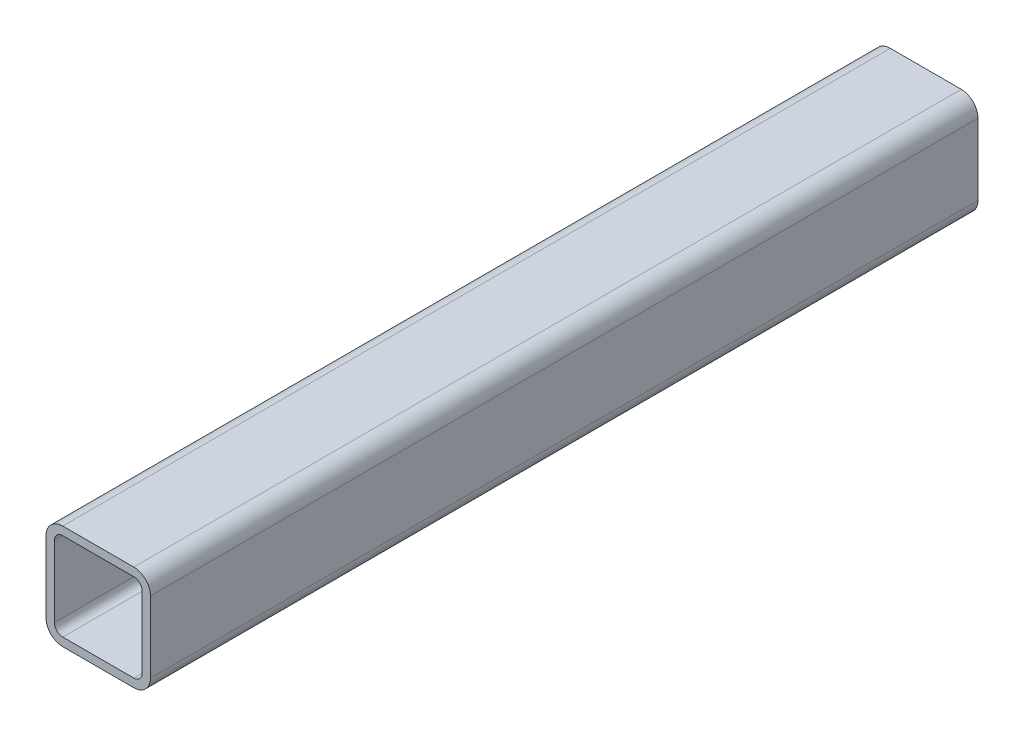
SolidWorks part; units mm, degrees
material "Q235"
ref_plane "Plane1" through (0, 0, 0) normal (0, 0, 1) x (1, 0, 0)
ref_plane "Plane2" through (0, 0, 0) normal (0, 1, 0) x (1, 0, 0)
ref_plane "Plane3" through (0, 0, 0) normal (1, 0, 0) x (0, 0, -1)
sketch "Sketch1" plane through (0, 0, 0) normal (0, 0, 1) x (1, 0, 0)
  line L0 (-8.5, -10.5) -> (8.5, -10.5)
  line L1 (-10.5, -8.5) -> (-10.5, 8.5)
  line L2 (8.5, 10.5) -> (-8.5, 10.5)
  line L3 (10.5, 8.5) -> (10.5, -8.5)
  line L4 (-8.5, -12.5) -> (8.5, -12.5)
  line L5 (-12.5, -8.5) -> (-12.5, 8.5)
  line L6 (8.5, 12.5) -> (-8.5, 12.5)
  line L7 (12.5, 8.5) -> (12.5, -8.5)
  arc A0 (12.5, 8.5) -> (8.5, 12.5) centre (8.5, 8.5) ccw
  arc A1 (8.5, -12.5) -> (12.5, -8.5) centre (8.5, -8.5) ccw
  arc A2 (-12.5, -8.5) -> (-8.5, -12.5) centre (-8.5, -8.5) ccw
  arc A3 (-8.5, 12.5) -> (-12.5, 8.5) centre (-8.5, 8.5) ccw
  arc A4 (-8.5, 10.5) -> (-10.5, 8.5) centre (-8.5, 8.5) ccw
  arc A5 (10.5, 8.5) -> (8.5, 10.5) centre (8.5, 8.5) ccw
  arc A6 (8.5, -10.5) -> (10.5, -8.5) centre (8.5, -8.5) ccw
  arc A7 (-10.5, -8.5) -> (-8.5, -10.5) centre (-8.5, -8.5) ccw
  point P0 (0, 12.5)
  point P1 (12.5, 0)
  point P2 (0, -12.5)
  point P3 (-12.5, 0)
  point P4 (-12.5, 12.5)
  point P5 (12.5, 12.5)
  point P6 (12.5, -12.5)
  point P7 (-12.5, -12.5)
  point P8 (0, 0)
extrude "Boss-Extrude1" add sketch "Sketch1" along normal blind 198
